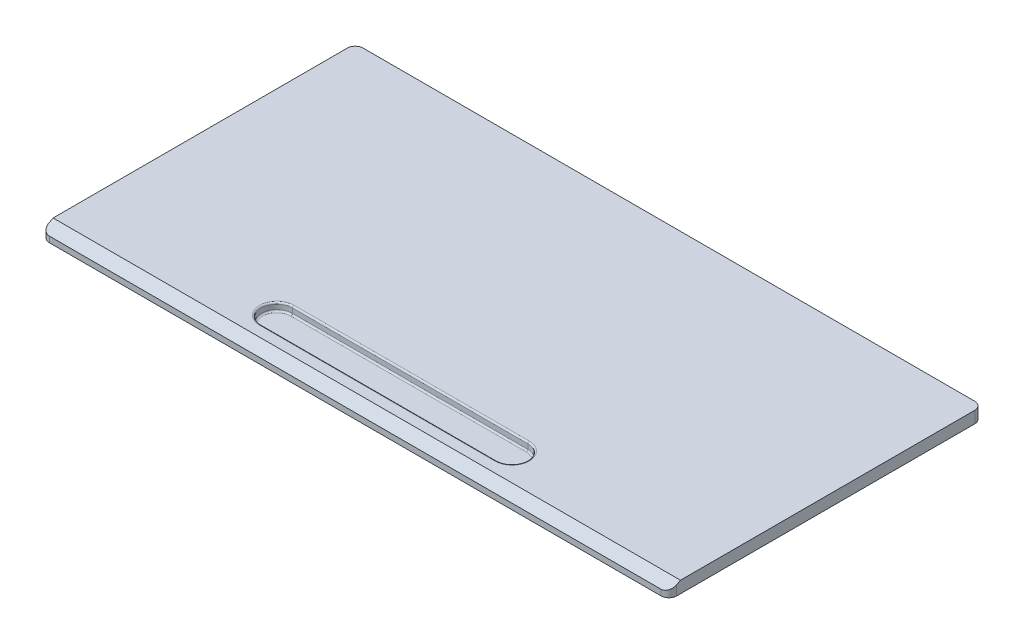
from build123d import *

# Parameters (mm, degrees)
SKETCH1_W           = 800
SKETCH1_H           = 400
BOSS_EXTRUDE1_DEPTH = 15
DRAFT1_ANGLE        = 1
FILLET1_R           = 10
CUT_EXTRUDE1_DEPTH  = 900
CUT_EXTRUDE2_DEPTH  = 10
FILLET2_R           = 2
SKETCH4_W           = 250
SKETCH4_H           = 15
BOSS_EXTRUDE2_DEPTH = 25
CUT_EXTRUDE4_DEPTH  = 10
SKETCH8_W           = 87.746039113
SKETCH8_H           = 29.522031851
BOSS_EXTRUDE3_DEPTH = 25
SKETCH9_R           = 5
CUT_EXTRUDE5_DEPTH  = 700


with BuildPart() as part:
    # Sketch1 → Boss-Extrude1 (new body)
    with BuildSketch(Plane(origin=(0, 0, 0), x_dir=(1, 0, 0), z_dir=(0, 1, 0))):
        Rectangle(SKETCH1_W, SKETCH1_H)
    extrude(amount=-BOSS_EXTRUDE1_DEPTH)

    # Draft1
    draft1_faces = [part.faces().sort_by_distance(p)[0] for p in [
        (0, -7.5, 200),
    ]]
    draft(draft1_faces, Plane(origin=(0, -15, 0), x_dir=(0, 0, -1), z_dir=(0, -1, 0)), DRAFT1_ANGLE)

    # Fillet1
    fillet1_edges = [part.edges().sort_by_distance(p)[0] for p in [
        (400, -7.5, 200.130912987),
        (-400, -7.5, 200.130912987),
        (-400, -7.5, -200),
        (400, -7.5, -200),
    ]]
    fillet(fillet1_edges, radius=FILLET1_R)

    # Sketch2 → Cut-Extrude1 (cut)
    with BuildSketch(Plane.ZY.offset(400)):
        Polygon((185.261825974, 0), (200.130912987, -7.5), (200.261825974, 0), align=None)
    extrude(amount=-CUT_EXTRUDE1_DEPTH, mode=Mode.SUBTRACT)

    # Sketch3 → Cut-Extrude2 (cut)
    with BuildSketch(Plane(origin=(0, 0, 0), x_dir=(1, 0, 0), z_dir=(0, 1, 0))):
        with BuildLine():
            Line((-150, -130), (150, -130))
            ThreePointArc((150, -130), (170, -150), (150, -170))
            Line((150, -170), (-150, -170))
            ThreePointArc((-150, -170), (-170, -150), (-150, -130))
        make_face()
    extrude(amount=-CUT_EXTRUDE2_DEPTH, mode=Mode.SUBTRACT)

    # Fillet2
    fillet2_edges = [part.edges().sort_by_distance(p)[0] for p in [
        (-170, -10, 150),
        (0, -10, 130),
        (170, -10, 150),
        (0, -10, 170),
        (-170, 0, 150),
        (0, 0, 170),
        (170, 0, 150),
        (0, 0, 130),
    ]]
    fillet(fillet2_edges, radius=FILLET2_R)

    # Sketch4 → Boss-Extrude2 (add)
    with BuildSketch(Plane.XZ.offset(15)):
        with Locations((-230, 66.25)):
            Rectangle(SKETCH4_W, SKETCH4_H)
    boss_extrude2 = extrude(amount=BOSS_EXTRUDE2_DEPTH)

    # Sketch7 → Cut-Extrude4 (cut)
    with BuildSketch(Plane(origin=(0, 0, 58.75), x_dir=(-1, 0, 0), z_dir=(0, 0, -1))):
        with BuildLine():
            Line((335, -33.5), (125, -33.5))
            ThreePointArc((125, -33.5), (119, -27.5), (125, -21.5))
            Line((125, -21.5), (335, -21.5))
            ThreePointArc((335, -21.5), (341, -27.5), (335, -33.5))
        make_face()
    cut_extrude4 = extrude(amount=-CUT_EXTRUDE4_DEPTH, mode=Mode.SUBTRACT)

    # Mirror2: Boss-Extrude2, Cut-Extrude4 across plane
    add(boss_extrude2.mirror(Plane.XY.offset(-36.25)))
    add(cut_extrude4.mirror(Plane.XY.offset(-36.25)), mode=Mode.SUBTRACT)

    # Sketch8 → Boss-Extrude3 (add)
    with BuildSketch(Plane.XZ.offset(15)):
        with Locations((310.696102603, 94.974826804)):
            Rectangle(SKETCH8_W, SKETCH8_H)
    boss_extrude3 = extrude(amount=BOSS_EXTRUDE3_DEPTH)

    # Mirror3: Boss-Extrude3 across plane
    add(boss_extrude3.mirror(Plane(origin=(0, 0, -36), x_dir=(1, 0, 0), z_dir=(0, 0, -1))))

    # Sketch9 → Cut-Extrude5 (cut)
    with BuildSketch(Plane(origin=(0, 0, -181.735842729), x_dir=(-1, 0, 0), z_dir=(0, 0, -1))):
        with Locations((-344.56912216, -27.5)):
            Circle(SKETCH9_R)
    extrude(amount=-CUT_EXTRUDE5_DEPTH, mode=Mode.SUBTRACT)


solid = part.part
